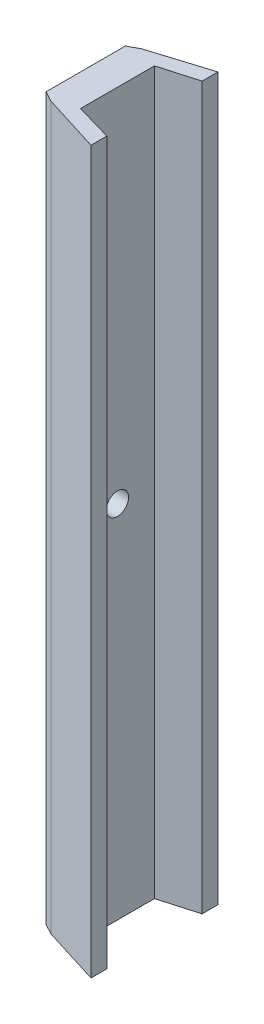
SolidWorks part; units mm, degrees
material "ZG270-500"
ref_plane "Front Plane" through (0, 0, 0) normal (0, 0, 1) x (1, 0, 0)
ref_plane "Top Plane" through (0, 0, 0) normal (0, 1, 0) x (1, 0, 0)
ref_plane "Right Plane" through (0, 0, 0) normal (1, 0, 0) x (0, 0, -1)
sketch "Sketch1" plane through (0, 0, 0) normal (0, 1, 0) x (1, 0, 0)
  line L0 (0, 0) -> (40.9343, 0) construction
  line L1 (0, -37.5) -> (0, 37.5)
  line L2 (0, 37.5) -> (10, 42.8818)
  line L3 (10, 42.8818) -> (65, 60)
  line L4 (65, 60) -> (65, 45)
  line L5 (65, 45) -> (30, 35)
  line L6 (30, 35) -> (30, -35)
  line L7 (65, -45) -> (30, -35)
  line L8 (65, -60) -> (65, -45)
  line L9 (10, -42.8818) -> (65, -60)
  line L10 (0, -37.5) -> (10, -42.8818)
  point P10 (30, 0)
  dimension "D1" = 11
  dimension "D2" = 70
  dimension "D3" = 90
  dimension "D4" = 120
  dimension "D5" = 30
  dimension "D6" = 65
  dimension "D7" = 75
  dimension "D8" = 10
extrude "Boss-Extrude1" add sketch "Sketch1" along normal mid plane 682
sketch "Sketch2" plane through (0, 0, 0) normal (-1, 0, 0) x (0, 0, 1)
  circle A0 centre (0, 0) radius 10.5
  dimension "D1" = 21
extrude "Cut-Extrude1" cut sketch "Sketch2" against normal blind 95
